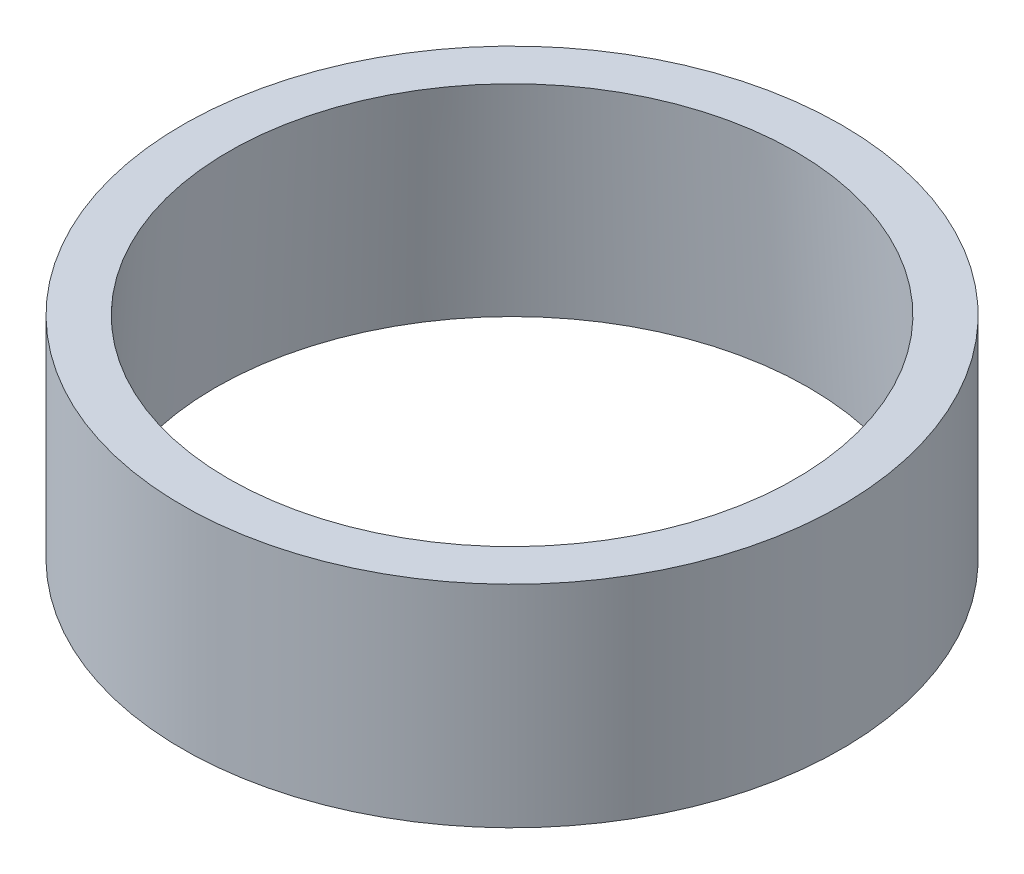
from build123d import *


with BuildPart() as part:
    # Sketch2 → Revolve1 (revolve)
    with BuildSketch(Plane.XY, mode=Mode.PRIVATE) as revolve1_sk:
        Polygon((43, 32), (45, 0), (50, 0), (50, 32), align=None)
    revolve(revolve1_sk.sketch.rotate(Axis((0, 0, 0), (0, 1, 0)), 90), axis=Axis((0, 0, 0), (0, 1, 0)))


solid = part.part
